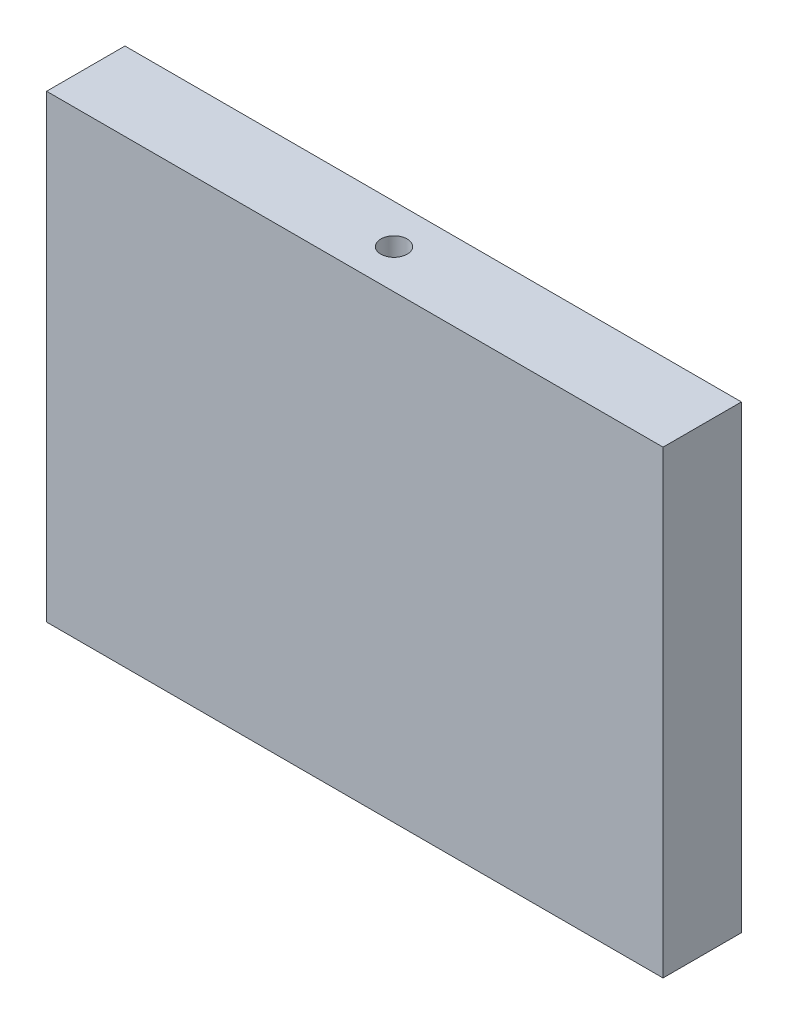
from build123d import *

# Parameters (mm, degrees)
SKETCH1_W           = 236
SKETCH1_H           = 176
BOSS_EXTRUDE1_DEPTH = 30
SKETCH3_R           = 5.055
CUT_EXTRUDE1_DEPTH  = 215.00934559


with BuildPart() as part:
    # Sketch1 → Boss-Extrude1 (new body)
    with BuildSketch(Plane.XY):
        Rectangle(SKETCH1_W, SKETCH1_H)
    extrude(amount=BOSS_EXTRUDE1_DEPTH)

    # Sketch3 → Cut-Extrude1 (cut, through all)
    with BuildSketch(Plane(origin=(0, 88, 0), x_dir=(1, 0, 0), z_dir=(0, 1, 0))):
        with Locations(Location((0, -15, 0), (0, 0, 180))):
            Circle(SKETCH3_R)
    extrude(amount=-CUT_EXTRUDE1_DEPTH, mode=Mode.SUBTRACT)


solid = part.part
